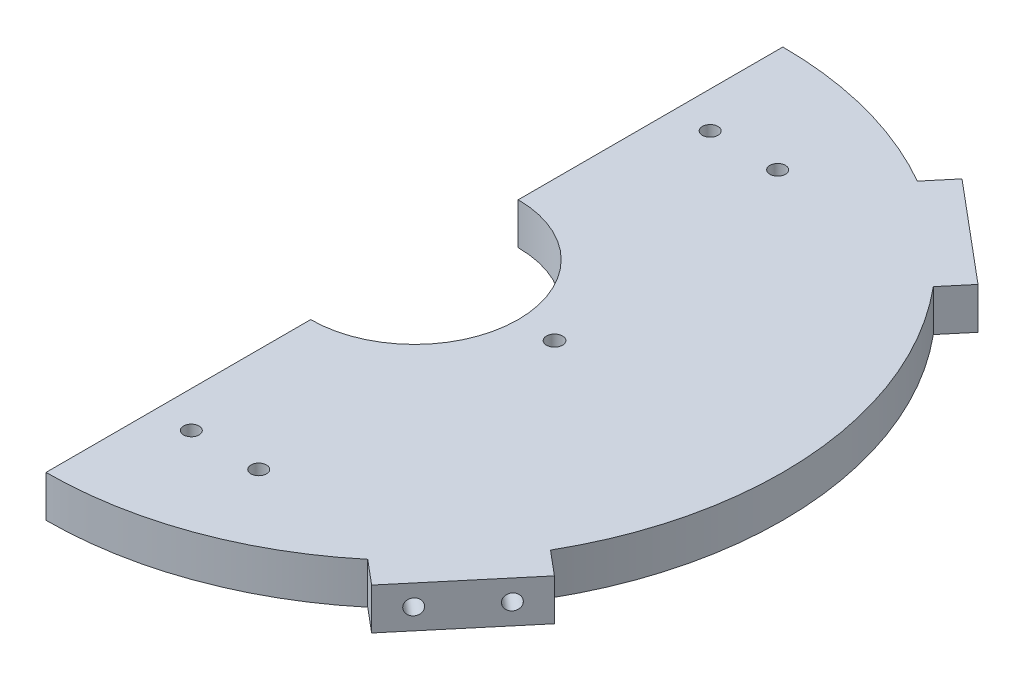
from build123d import *

# Parameters (mm, degrees)
BOSS_EXTRUDE1_DEPTH = 8
SKETCH2_R           = 1.5
CUT_EXTRUDE1_DEPTH  = 101.727354775
BOSS_EXTRUDE2_START = -71
SKETCH3_W           = 8
SKETCH3_H           = 25
BOSS_EXTRUDE2_DEPTH = 5
SKETCH4_R           = 1.5
CUT_EXTRUDE2_DEPTH  = 5
CIRPATTERN1_COUNT   = 2
CIRPATTERN1_ANGLE   = 90
SKETCH5_R           = 1.55
CUT_EXTRUDE3_DEPTH  = 101.727354775


with BuildPart() as part:
    # Sketch1 → Boss-Extrude1 (new body)
    with BuildSketch(Plane(origin=(0, 0, 0), x_dir=(1, 0, 0), z_dir=(0, 1, 0))):
        with BuildLine():
            Line((0, -71), (0, -20))
            ThreePointArc((0, -20), (20, 0), (0, 20))
            Line((0, 20), (0, 71))
            ThreePointArc((0, 71), (71, 0), (0, -71))
        make_face()
    extrude(amount=BOSS_EXTRUDE1_DEPTH)

    # Sketch2 → Cut-Extrude1 (cut, through all)
    with BuildSketch(Plane(origin=(0, 8, 0), x_dir=(1, 0, 0), z_dir=(0, 1, 0))):
        with Locations(Location((7, 50, 0), (0, 0, 270))):
            Circle(SKETCH2_R)
        with Locations(Location((20, 50, 0), (0, 0, 270))):
            Circle(SKETCH2_R)
        with Locations(Location((20, -50, 0), (0, 0, 90))):
            Circle(SKETCH2_R)
        with Locations(Location((7, -50, 0), (0, 0, 90))):
            Circle(SKETCH2_R)
    extrude(amount=-CUT_EXTRUDE1_DEPTH, mode=Mode.SUBTRACT)

    # Sketch3 → Boss-Extrude2 (add, symmetric)
    with BuildSketch(Plane(origin=(0, 0, 0), x_dir=(0, -1, 0), z_dir=(-0.6427876096865403, 0, 0.7660444431189772)).offset(BOSS_EXTRUDE2_START)):
        with Locations((-4, 0)):
            Rectangle(SKETCH3_W, SKETCH3_H)
    boss_extrude2 = extrude(amount=BOSS_EXTRUDE2_DEPTH, both=True)

    # Sketch4 → Cut-Extrude2 (cut)
    with BuildSketch(Plane(origin=(48.851858336, 0, -58.219377677), x_dir=(-0.7660444431189771, 0, -0.6427876096865404), z_dir=(0.6427876096865404, 0, -0.7660444431189771))):
        with Locations((-6.75, 4)):
            Circle(SKETCH4_R)
        with Locations((6.75, 4)):
            Circle(SKETCH4_R)
    cut_extrude2 = extrude(amount=-CUT_EXTRUDE2_DEPTH, mode=Mode.SUBTRACT)

    # CirPattern1: Boss-Extrude2, Cut-Extrude2 ×2 about axis
    cirpattern1_axis = Axis((0, 0, 0), (0, -1, 0))
    add([boss_extrude2.rotate(cirpattern1_axis, i * CIRPATTERN1_ANGLE / (CIRPATTERN1_COUNT - 1)) for i in range(1, CIRPATTERN1_COUNT)])
    add([cut_extrude2.rotate(cirpattern1_axis, i * CIRPATTERN1_ANGLE / (CIRPATTERN1_COUNT - 1)) for i in range(1, CIRPATTERN1_COUNT)], mode=Mode.SUBTRACT)

    # Sketch5 → Cut-Extrude3 (cut, through all)
    with BuildSketch(Plane(origin=(0, 8, 0), x_dir=(1, 0, 0), z_dir=(0, 1, 0))):
        with Locations(Location((27, 0, 0), (0, 0, 270))):
            Circle(SKETCH5_R)
    extrude(amount=-CUT_EXTRUDE3_DEPTH, mode=Mode.SUBTRACT)


solid = part.part
